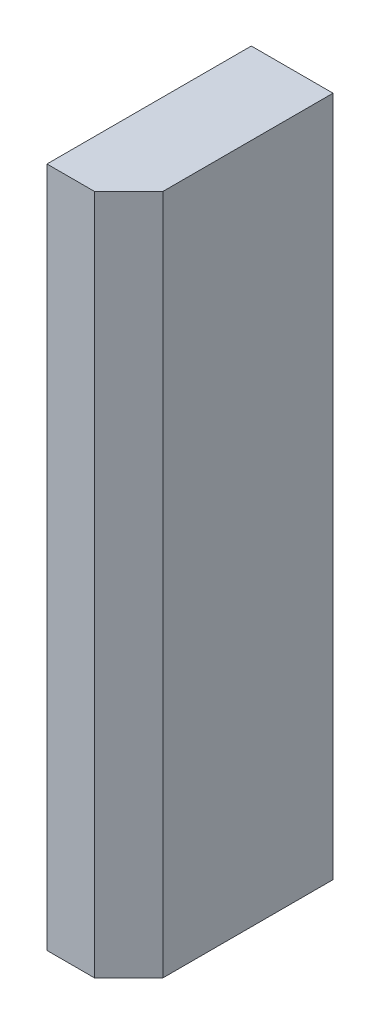
from build123d import *

# Parameters (mm, degrees)
SKETCH1_W           = 120
SKETCH1_H           = 1000
BOSS_EXTRUDE1_DEPTH = 300
CHAMFER1_SIZE       = 50


with BuildPart() as part:
    # Sketch1 → Boss-Extrude1 (new body)
    with BuildSketch(Plane.XY):
        Rectangle(SKETCH1_W, SKETCH1_H)
    extrude(amount=BOSS_EXTRUDE1_DEPTH)

    # Chamfer1
    chamfer1_edges = [part.edges().sort_by_distance(p)[0] for p in [
        (60, 0, 300),
    ]]
    chamfer(chamfer1_edges, length=CHAMFER1_SIZE)


solid = part.part
